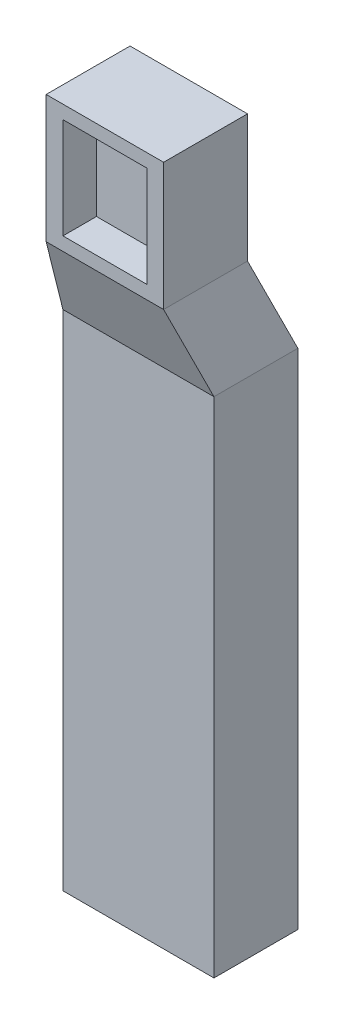
SolidWorks part; units mm, degrees
ref_plane "Front Plane" through (0, 0, 0) normal (0, 0, 1) x (1, 0, 0)
ref_plane "Top Plane" through (0, 0, 0) normal (0, 1, 0) x (1, 0, 0)
ref_plane "Right Plane" through (0, 0, 0) normal (1, 0, 0) x (0, 0, -1)
other "Configuration Table"
sketch "Sketch2" plane through (0, 0, 0) normal (0, 0, 1) x (1, 0, 0)
  line L0 (0, 0) -> (0, -1190) construction
  line L1 (-175, 190) -> (175, 190)
  line L2 (-175, 190) -> (-175, -190)
  line L3 (-175, -190) -> (175, -190) construction
  line L4 (175, 190) -> (175, -190)
  line L5 (-175, 190) -> (175, -190) construction
  line L6 (-175, -190) -> (175, 190) construction
  line L7 (-225, -440) -> (225, -440) construction
  line L8 (-225, -440) -> (-225, -1940)
  line L9 (-225, -1940) -> (225, -1940)
  line L10 (225, -440) -> (225, -1940)
  line L11 (-225, -440) -> (225, -1940) construction
  line L12 (-225, -1940) -> (225, -440) construction
  line L13 (-175, -190) -> (-225, -440)
  line L14 (175, -190) -> (225, -440)
  point P0 (0, 0)
  point P6 (0, -1190)
  dimension "D1" = 350
  dimension "D2" = 380
  dimension "D3" = 250
  dimension "D4" = 450
  dimension "D5" = 1500
extrude "Boss-Extrude1" add sketch "Sketch2" along normal blind 350
sketch "Sketch3" plane through (-225, 0, 0) normal (-1, 0, 0) x (0, 0, 1)
  line L0 (350, -190) -> (250, -440)
  line L1 (350, -440) -> (0, -440) construction
  line L2 (250, -440) -> (250, -1940)
  line L3 (350, -1940) -> (0, -1940) construction
  line L4 (250, -1940) -> (350, -1940)
  line L5 (350, -1940) -> (350, -190)
  line L10 (0, -440) -> (100, -190)
  line L11 (350, -190) -> (0, -190) construction
  line L12 (100, -190) -> (100, 190)
  line L13 (350, 190) -> (0, 190) construction
  line L14 (100, 190) -> (0, 190)
  line L15 (0, 190) -> (0, -440)
  dimension "D1" = 100
  dimension "D2" = 100
extrude "Cut-Extrude1" cut sketch "Sketch3" against normal through all
sketch "Sketch4" plane through (0, 0, 350) normal (0, 0, 1) x (1, 0, 0)
  line L0 (-175, 190) -> (175, -190) construction
  line L2 (-125, 150) -> (125, 150)
  line L3 (-125, 150) -> (-125, -150)
  line L4 (-125, -150) -> (125, -150)
  line L5 (125, 150) -> (125, -150)
  line L6 (-125, 150) -> (125, -150) construction
  line L7 (-125, -150) -> (125, 150) construction
  point P4 (0, 0)
  dimension "D1" = 300
  dimension "D2" = 250
extrude "Cut-Extrude2" cut sketch "Sketch4" against normal blind 100
